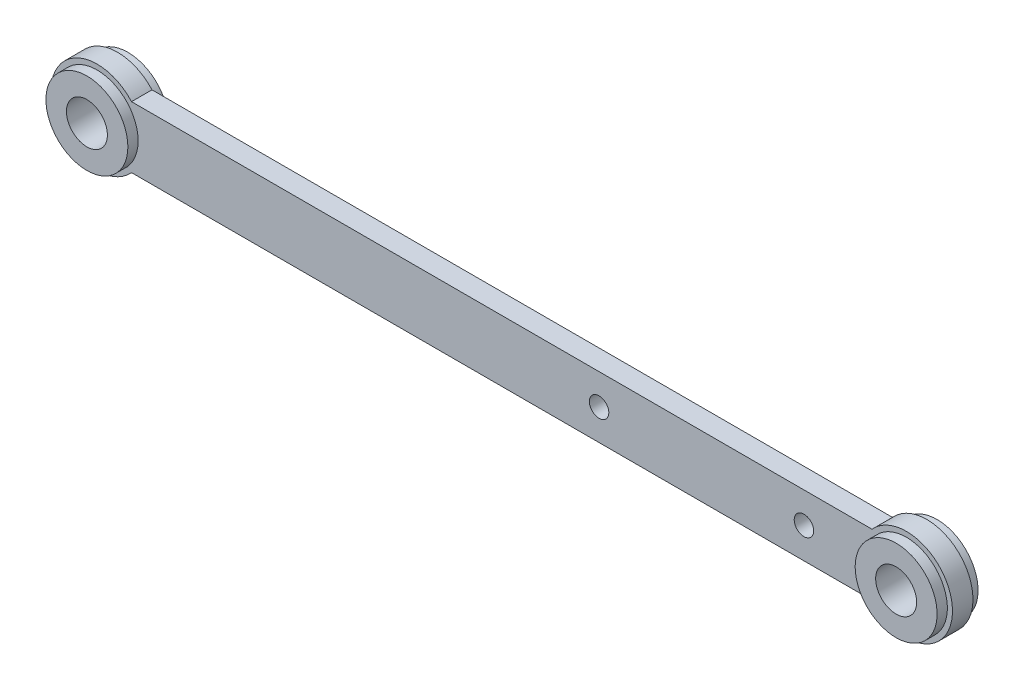
SolidWorks part; units mm, degrees
material "Q235A"
ref_plane "前视基准面" through (0, 0, 0) normal (0, 0, 1) x (1, 0, 0)
ref_plane "上视基准面" through (0, 0, 0) normal (0, 1, 0) x (1, 0, 0)
ref_plane "右视基准面" through (0, 0, 0) normal (1, 0, 0) x (0, 0, -1)
sketch "草图1" plane through (0, 0, 0) normal (0, 0, 1) x (1, 0, 0)
  line L1 (395, -30) -> (-395, -30)
  line L2 (395, -30) -> (395, 30)
  line L3 (395, 30) -> (-395, 30)
  line L4 (-395, -30) -> (-395, 30)
  line L5 (395, -30) -> (-395, 30) construction
  line L6 (395, 30) -> (-395, -30) construction
  circle A0 centre (-395, 0) radius 20
  circle A1 centre (-395, 0) radius 45
  circle A2 centre (395, 0) radius 45
  circle A3 centre (395, 0) radius 20
  point P0 (0, 0)
  dimension "D2" = 40
  dimension "D4" = 90
  dimension "D5" = 90
  dimension "D6" = 40
  dimension "D1" = 790
  dimension "D3" = 60
extrude "凸台-拉伸1" add sketch "草图1" along normal blind 20 contours A2 L3 A1 L1 | L4 A1 A0 | L4 A1 A0 | A3 L2 A2 | A3 L2 A2
sketch "草图2" plane through (0, 0, 20) normal (0, 0, 1) x (1, 0, 0)
  line L0 (0, 0) -> (0, -99.077) construction
  circle A0 centre (-395, 0) radius 20 construction
  circle A1 centre (-395, 0) radius 20
  circle A3 centre (-395, 0) radius 40
  arc A4 (-361.459, 30) -> (-361.459, -30) centre (-395, 0) ccw construction
  circle A5 centre (395, 0) radius 40
  circle A6 centre (395, 0) radius 20
  dimension "D1" = 5
extrude "凸台-拉伸2" add sketch "草图2" along normal blind 10
sketch "草图3" plane through (0, 0, 0) normal (0, 0, -1) x (-1, 0, 0)
  circle A1 centre (-395, 0) radius 20
  circle A2 centre (-395, 0) radius 20
  circle A3 centre (-395, 0) radius 40
  circle A4 centre (-395, 0) radius 40
  circle A5 centre (395, 0) radius 40
  circle A6 centre (395, 0) radius 40
  circle A7 centre (395, 0) radius 20
  circle A8 centre (395, 0) radius 20
  dimension "D1" = 0
  dimension "D2" = 0
  dimension "D3" = 0
  dimension "D4" = 0
extrude "凸台-拉伸3" add sketch "草图3" along normal blind 10
hole_wizard "M16 间隙孔1" positions "草图4" profile "草图5" hole size "M16" standard "ISO" end condition through all
sketch "草图4" plane through (0, 0, 20) normal (0, 0, 1) x (1, 0, 0)
  circle A0 centre (395, 0) radius 20 construction
  point P0 (95, 0)
  point P3 (295, 0)
  dimension "D1" = 200
  dimension "D2" = 100
sketch "草图5" plane through (95, 0, 20) normal (1, 0, 0) x (0, -1, 0)
  line L0 (0, 0) -> (0, 30)
  line L1 (0, 30) -> (9.5, 30)
  line L2 (9.5, 30) -> (9.5, 0)
  line L5 (9.5, 0) -> (0, 0)
  line L11 (0, -6.35) -> (0, 107.95) construction
  dimension "通孔孔直径" = 19
  dimension "通孔孔深度" = 30
